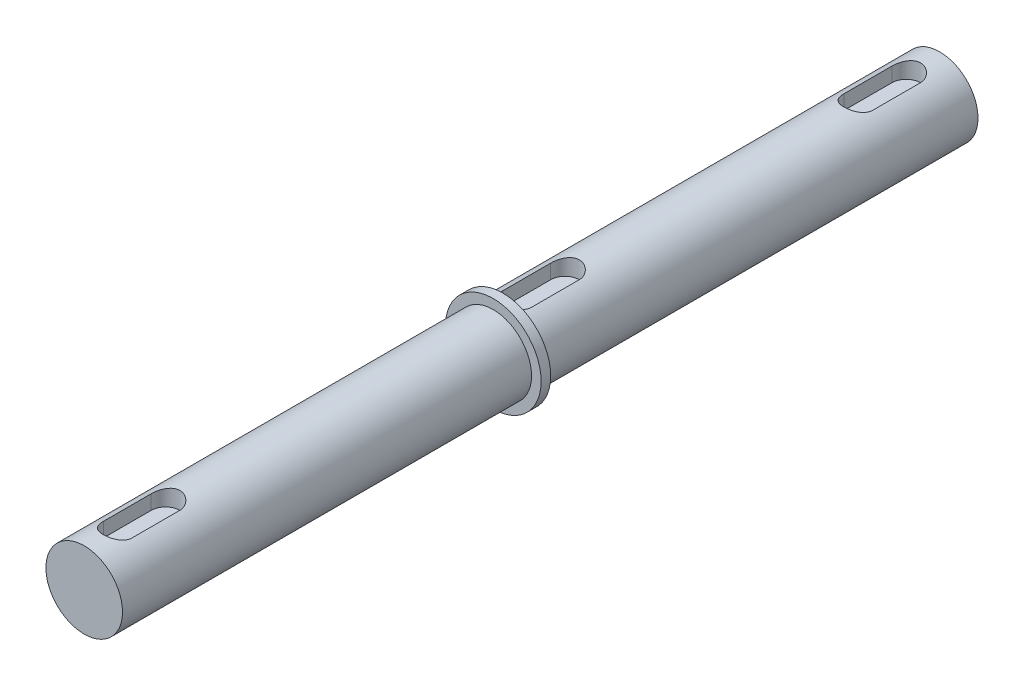
SolidWorks part; units mm, degrees
ref_plane "Front Plane" through (0, 0, 0) normal (0, 0, 1) x (1, 0, 0)
ref_plane "Top Plane" through (0, 0, 0) normal (0, 1, 0) x (1, 0, 0)
ref_plane "Right Plane" through (0, 0, 0) normal (1, 0, 0) x (0, 0, -1)
other "Configuration Table"
sketch "Sketch1" plane through (0, 0, 0) normal (0, 0, 1) x (1, 0, 0)
  circle A0 centre (0, 0) radius 4
  dimension "D1" = 8
extrude "Boss-Extrude1" add sketch "Sketch1" along normal blind 45.65
sketch "Sketch2" plane through (0, 0, 45.65) normal (0, 0, 1) x (1, 0, 0)
  circle A0 centre (0, 0) radius 5
  dimension "D1" = 10
extrude "Boss-Extrude2" add sketch "Sketch2" along normal blind 1
sketch "Sketch3" plane through (0, 0, 46.65) normal (0, 0, 1) x (1, 0, 0)
  circle A0 centre (0, 0) radius 4
  dimension "D1" = 8
extrude "Boss-Extrude3" add sketch "Sketch3" along normal blind 42.74
ref_plane "Plane1" through (0, 4, 0) normal (0, 1, 0) x (1, 0, 0)
sketch "Sketch4" plane through (0, 4, 0) normal (0, 1, 0) x (1, 0, 0)
  line L0 (-4, -89.39) -> (4, -89.39) construction
  line L2 (5, -45.65) -> (-5, -45.65) construction
  line L3 (-4, -89.39) -> (4, -89.39) construction
  line L4 (0, -121.2644) -> (0, 121.2644) construction
  line L5 (5, -45.65) -> (-5, -45.65) construction
  line L6 (0, -3.5) -> (0, -8.5) construction
  line L7 (1.5, -3.5) -> (1.5, -8.5)
  line L8 (-1.5, -3.5) -> (-1.5, -8.5)
  line L9 (4, 0) -> (-4, 0) construction
  line L10 (0, -39.15) -> (0, -44.15) construction
  line L11 (1.5, -39.15) -> (1.5, -44.15)
  line L12 (-1.5, -39.15) -> (-1.5, -44.15)
  line L13 (0, -80.89) -> (0, -85.89) construction
  line L14 (1.5, -80.89) -> (1.5, -85.89)
  line L15 (-1.5, -80.89) -> (-1.5, -85.89)
  arc A0 (1.5, -3.5) -> (-1.5, -3.5) centre (0, -3.5) ccw
  arc A1 (-1.5, -8.5) -> (1.5, -8.5) centre (0, -8.5) ccw
  arc A2 (1.5, -39.15) -> (-1.5, -39.15) centre (0, -39.15) ccw
  arc A3 (-1.5, -44.15) -> (1.5, -44.15) centre (0, -44.15) ccw
  arc A4 (1.5, -80.89) -> (-1.5, -80.89) centre (0, -80.89) ccw
  arc A5 (-1.5, -85.89) -> (1.5, -85.89) centre (0, -85.89) ccw
  point P8 (0, 0)
  point P11 (0, -6)
  point P20 (0, -41.65)
  point P27 (0, -83.39)
  dimension "D2" = 1.5
  dimension "D5" = 1.5
  dimension "D7" = 1.5
  dimension "D1" = 5
  dimension "D3" = 3.5
  dimension "D4" = 5
  dimension "D6" = 1.5
  dimension "D8" = 5
  dimension "D9" = 3.5
extrude "Cut-Extrude1" cut sketch "Sketch4" against normal blind 1.8
